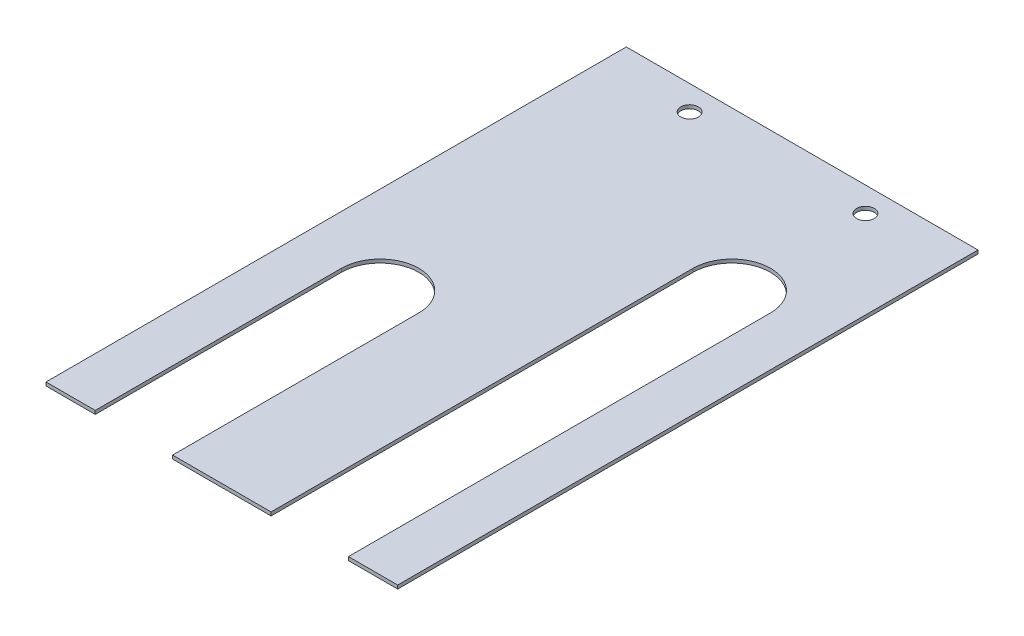
SolidWorks part; units mm, degrees
material "A3"
ref_plane "前视基准面" through (0, 0, 0) normal (0, 0, 1) x (1, 0, 0)
ref_plane "上视基准面" through (0, 0, 0) normal (0, 1, 0) x (1, 0, 0)
ref_plane "右视基准面" through (0, 0, 0) normal (1, 0, 0) x (0, 0, -1)
sketch "草图1" plane through (0, 0, 0) normal (0, 1, 0) x (1, 0, 0)
  line L1 (-50, -82.5) -> (50, -82.5)
  line L2 (-50, -82.5) -> (-50, 82.5)
  line L3 (-50, 82.5) -> (50, 82.5)
  line L4 (50, -82.5) -> (50, 82.5)
  line L5 (-50, -82.5) -> (50, 82.5) construction
  line L6 (-50, 82.5) -> (50, -82.5) construction
  point P0 (0, 0)
  dimension "D1" = 165
  dimension "D2" = 100
extrude "凸台-拉伸1" add sketch "草图1" along normal blind 1
sketch "草图2" plane through (0, 1, 0) normal (0, 1, 0) x (1, 0, 0)
  line L0 (-25, -82.5) -> (-25, -12.5) construction
  line L1 (-50, -82.5) -> (50, -82.5) construction
  line L2 (-36, -82.5) -> (-36, -12.5)
  line L3 (-14, -82.5) -> (-14, -12.5)
  line L4 (25, -82.5) -> (25, 37.5) construction
  line L5 (14, -82.5) -> (14, 37.5)
  line L6 (36, -82.5) -> (36, 37.5)
  line L7 (50, 82.5) -> (-50, 82.5) construction
  arc A0 (-36, -82.5) -> (-14, -82.5) centre (-25, -82.5) ccw
  arc A1 (-14, -12.5) -> (-36, -12.5) centre (-25, -12.5) ccw
  arc A2 (14, -82.5) -> (36, -82.5) centre (25, -82.5) ccw
  arc A3 (36, 37.5) -> (14, 37.5) centre (25, 37.5) ccw
  circle A4 centre (-25, 75.5) radius 2.5
  circle A5 centre (25, 75.5) radius 2.5
  point P4 (-25, -47.5)
  point P9 (25, -22.5)
  dimension "D1" = 11
  dimension "D2" = 11
  dimension "D7" = 5
  dimension "D8" = 7
  dimension "D3" = 45
  dimension "D4" = 25
  dimension "D5" = 25
  dimension "D6" = 50
extrude "切除-拉伸1" cut sketch "草图2" against normal through all
